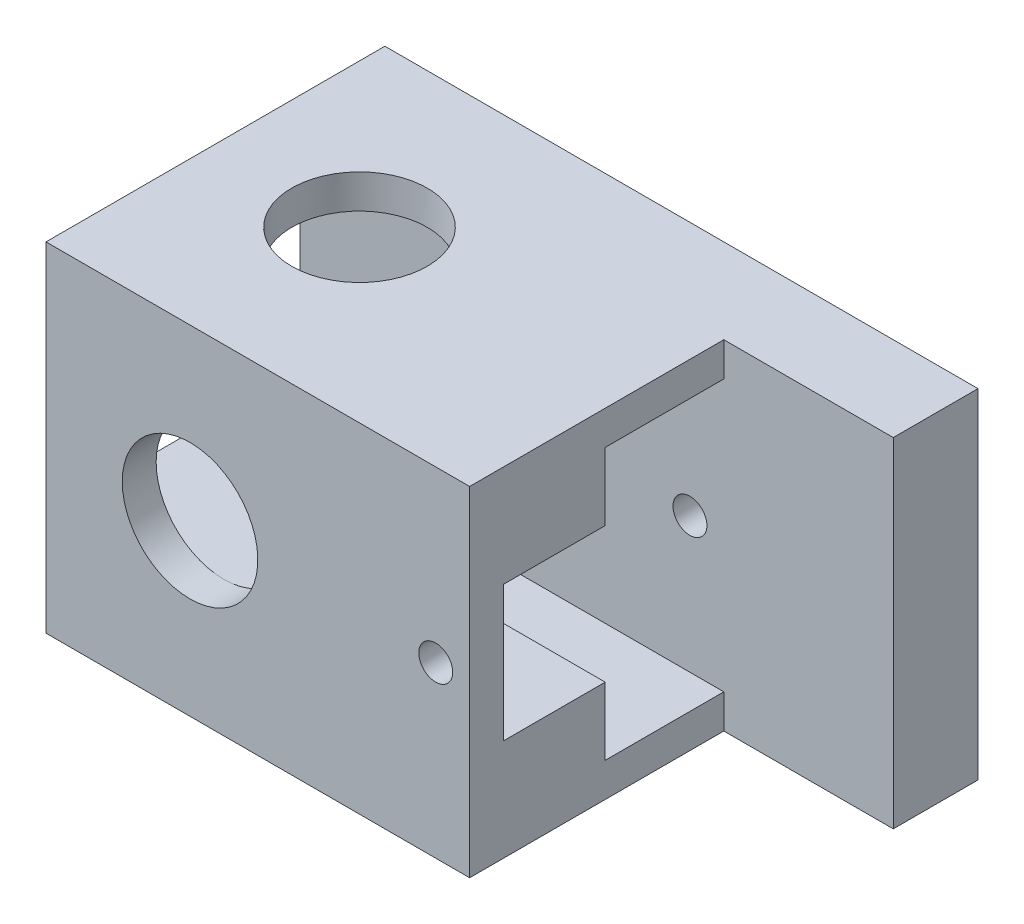
SolidWorks part; units mm, degrees
ref_plane "Front Plane" through (0, 0, 0) normal (0, 0, 1) x (1, 0, 0)
ref_plane "Top Plane" through (0, 0, 0) normal (0, 1, 0) x (1, 0, 0)
ref_plane "Right Plane" through (0, 0, 0) normal (1, 0, 0) x (0, 0, -1)
other "Configuration Table"
sketch "Sketch1" plane through (0, 0, 0) normal (0, 1, 0) x (1, 0, 0)
  line L0 (0, 0) -> (25, 0)
  line L1 (25, 0) -> (25, 15)
  line L2 (25, 15) -> (35, 15)
  line L3 (35, 15) -> (35, 20)
  line L4 (35, 20) -> (0, 20)
  line L5 (0, 20) -> (0, 0)
  dimension "D1" = 20
  dimension "D2" = 25
  dimension "D3" = 15
  dimension "D4" = 10
extrude "Boss-Extrude1" add sketch "Sketch1" along normal blind 20
sketch "Sketch2" plane through (0, 0, 0) normal (0, 0, 1) x (1, 0, 0)
  line L0 (8.5, 20) -> (8.5, 0) construction
  line L1 (0, 20) -> (25, 20) construction
  line L2 (12.5, 20) -> (12.5, 0) construction
  line L3 (0, 0) -> (25, 0) construction
  line L4 (25, 20) -> (25, 0) construction
  circle A0 centre (8.5, 10) radius 4
  circle A1 centre (23, 10) radius 1
  dimension "D1" = 8
  dimension "D2" = 4
  dimension "D3" = 10
  dimension "D4" = 2
  dimension "D5" = 10
  dimension "D6" = 2
extrude "Cut-Extrude1" cut sketch "Sketch2" against normal through all both and the other way through all
sketch "Sketch5" plane through (0, 20, 0) normal (0, 1, 0) x (1, 0, 0)
  line L0 (12.5, 0) -> (12.5, 20) construction
  line L1 (0, 0) -> (25, 0) construction
  line L2 (35, 20) -> (0, 20) construction
  circle A0 centre (8.5, 10) radius 4
  dimension "D1" = 8
  dimension "D2" = 4
  dimension "D3" = 10
extrude "Cut-Extrude3" cut sketch "Sketch5" against normal through all both and the other way through all
sketch "Sketch6" plane through (25, 0, 0) normal (1, 0, 0) x (0, 0, -1)
  line L0 (2, 14) -> (2, 6)
  line L1 (2, 6) -> (8, 6)
  line L2 (8, 6) -> (8, 2.0046)
  line L3 (8, 2.0046) -> (15, 2.0046)
  line L4 (15, 20) -> (15, 0) construction
  line L5 (15, 2.0046) -> (15, 17.9954)
  line L8 (8, 17.9954) -> (15, 17.9954)
  line L9 (8, 14) -> (8, 17.9954)
  line L10 (2, 14) -> (8, 14)
  line L11 (0, 20) -> (15, 20) construction
  line L12 (0, 0) -> (15, 0) construction
  line L14 (0, 20) -> (0, 0) construction
  dimension "D1" = 2.0046
  dimension "D2" = 2.0046
  dimension "D3" = 6
  dimension "D4" = 8
  dimension "D5" = 6
  dimension "D6" = 8
  dimension "D7" = 2
extrude "Cut-Extrude4" cut sketch "Sketch6" against normal through all
